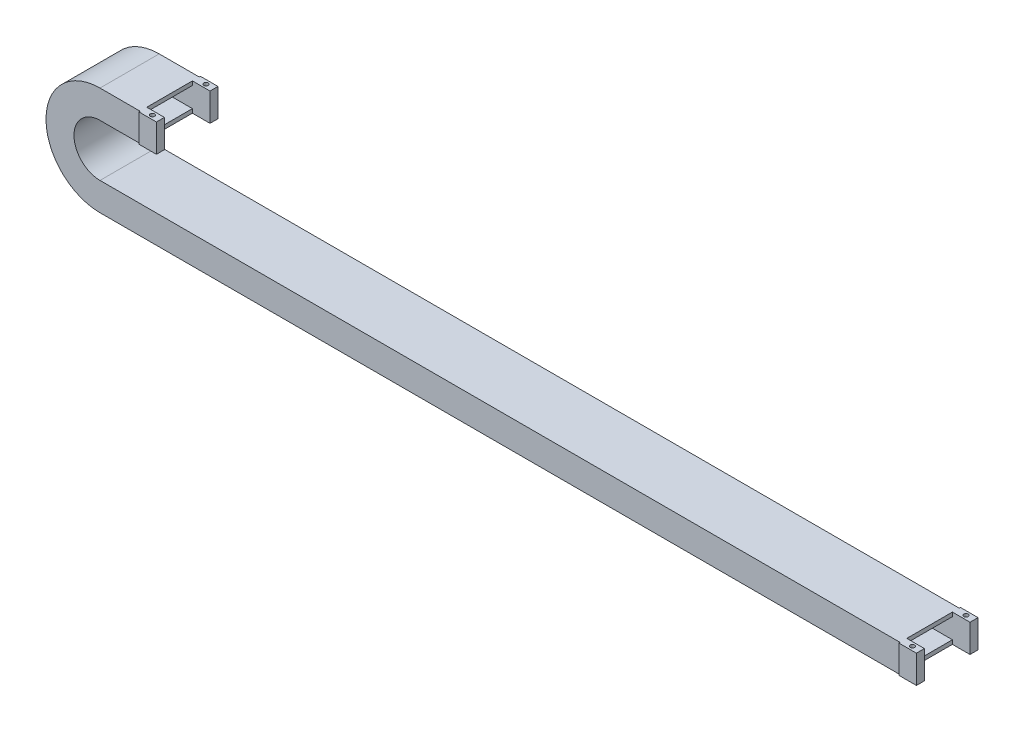
from build123d import *

# Parameters (mm, degrees)
SKETCH_2_W                  = 74
SKETCH_2_H                  = 35
SKETCH_2_W_2                = 57
SKETCH_2_H_2                = 25
SKETCH_11_W                 = 77
SKETCH_11_H                 = 35
SKETCH_11_W_2               = 57
SKETCH_11_H_2               = 25
EXTRUDE_1_DEPTH             = 22
SKETCH_12_W                 = 23.011901601
SKETCH_12_H                 = 57
CUT_EXTRUDE_9_DEPTH         = 1073.864623333
HOLE_WIZARD_5_5_5_5_1_D     = 5.5
SKETCH_15_W                 = 77
SKETCH_15_H                 = 35
SKETCH_15_W_2               = 57
SKETCH_15_H_2               = 25
EXTRUDE_2_DEPTH             = 22
SKETCH_16_W                 = 45.795478168
SKETCH_16_H                 = 57
CUT_EXTRUDE_10_DEPTH        = 49
HOLE_WIZARD_5_5_5_5_2_D     = 5.5
HOLE_WIZARD_5_5_5_5_2_DEPTH = 50
HOLE_WIZARD_5_5_5_5_2_TIP   = 1.652366702


with BuildPart() as part:
    # 扫描1: sweep along a path in 草图1
    with BuildLine(Plane.XY) as sweep_1_path:
        Line((0, 0), (-1000, 0))
        ThreePointArc((-1000, 0), (-1050, 50), (-1000, 100))
        Line((-1000, 100), (-950, 100))
    # 草图2 → 扫描1 (sweep)
    with BuildSketch(Plane(origin=(0, 0, 0), x_dir=(0, 0, -1), z_dir=(1, 0, 0))):
        Rectangle(SKETCH_2_W, SKETCH_2_H)
        Rectangle(SKETCH_2_W_2, SKETCH_2_H_2, mode=Mode.SUBTRACT)
    sweep(path=sweep_1_path.line)

    # 草图11 → 凸台-拉伸1 (add)
    with BuildSketch(Plane(origin=(0, 0, 0), x_dir=(0, 0, -1), z_dir=(1, 0, 0))):
        Rectangle(SKETCH_11_W, SKETCH_11_H)
        Rectangle(SKETCH_11_W_2, SKETCH_11_H_2, mode=Mode.SUBTRACT)
    extrude(amount=EXTRUDE_1_DEPTH)

    # 草图12 → 切除-拉伸9 (cut, through all)
    with BuildSketch(Plane(origin=(0, 17.5, 0), x_dir=(1, 0, 0), z_dir=(0, 1, 0))):
        with Locations((11.505950801, 0)):
            Rectangle(SKETCH_12_W, SKETCH_12_H)
    extrude(amount=-CUT_EXTRUDE_9_DEPTH, mode=Mode.SUBTRACT)

    # Ø5.5 (5.5) 直径孔1 (through all)
    with Locations(Plane(origin=(0, 17.5, 0), x_dir=(1, 0, 0), z_dir=(0, 1, 0))):
        with Locations((12, 33.5), (12, -33.5)):
            Hole(HOLE_WIZARD_5_5_5_5_1_D / 2)

    # 草图15 → 凸台-拉伸2 (add)
    with BuildSketch(Plane(origin=(-950, 0, 0), x_dir=(0, 0, -1), z_dir=(1, 0, 0))):
        with Locations((0, 100)):
            Rectangle(SKETCH_15_W, SKETCH_15_H)
        with Locations((0, 100)):
            Rectangle(SKETCH_15_W_2, SKETCH_15_H_2, mode=Mode.SUBTRACT)
    extrude(amount=EXTRUDE_2_DEPTH)

    # 草图16 → 切除-拉伸10 (cut)
    with BuildSketch(Plane(origin=(0, 117.5, 0), x_dir=(1, 0, 0), z_dir=(0, 1, 0))):
        with Locations((-927.102260916, 0)):
            Rectangle(SKETCH_16_W, SKETCH_16_H)
    extrude(amount=-CUT_EXTRUDE_10_DEPTH, mode=Mode.SUBTRACT)

    # Ø5.5 (5.5) 直径孔2
    with Locations(Plane(origin=(0, 117.5, 0), x_dir=(1, 0, 0), z_dir=(0, 1, 0))):
        with Locations((-938, 33.5), (-938, -33.5)):
            Hole(HOLE_WIZARD_5_5_5_5_2_D / 2, depth=HOLE_WIZARD_5_5_5_5_2_DEPTH)
            with Locations((0, 0, -(HOLE_WIZARD_5_5_5_5_2_DEPTH + HOLE_WIZARD_5_5_5_5_2_TIP / 2))):  # 118° drill point
                Cone(0, HOLE_WIZARD_5_5_5_5_2_D / 2, HOLE_WIZARD_5_5_5_5_2_TIP, mode=Mode.SUBTRACT)


solid = part.part
